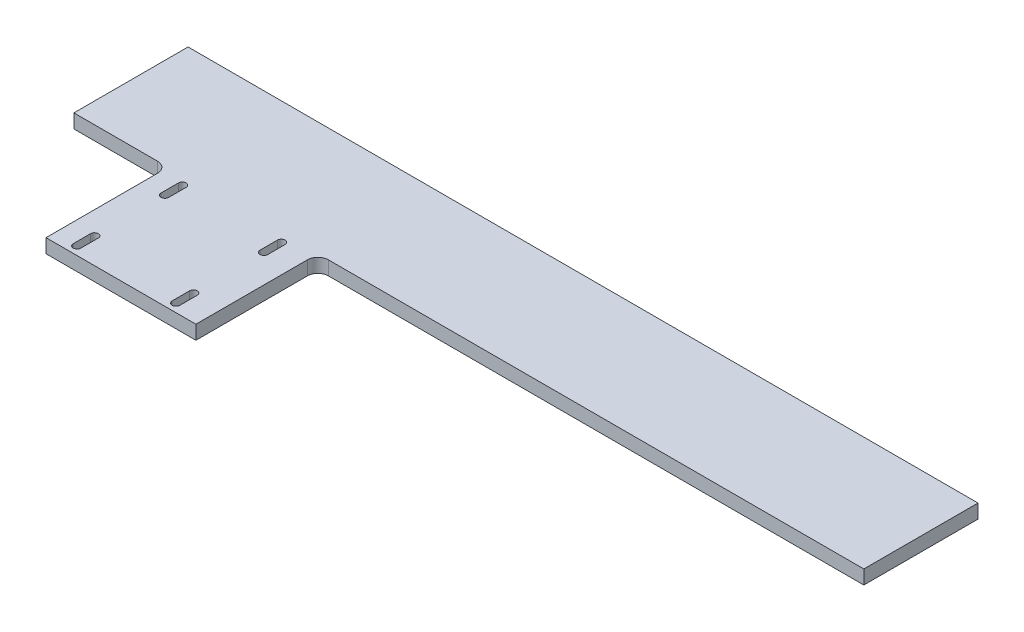
from build123d import *

# Parameters (mm, degrees)
SKETCH_1_W          = 2266
SKETCH_1_H          = 327.5
EXTRUDE_1_DEPTH     = 40
SKETCH_2_W          = 430
SKETCH_2_H          = 350
EXTRUDE_2_DEPTH     = 40
CUT_EXTRUDE_1_DEPTH = 1245.67990363
FILLET_1_R          = 30


with BuildPart() as part:
    # 草图1 → 凸台-拉伸1 (new body)
    with BuildSketch(Plane(origin=(0, 0, 0), x_dir=(1, 0, 0), z_dir=(0, 1, 0))):
        Rectangle(SKETCH_1_W, SKETCH_1_H)
    extrude(amount=EXTRUDE_1_DEPTH)

    # 草图2 → 凸台-拉伸2 (add)
    with BuildSketch(Plane(origin=(0, 40, 0), x_dir=(1, 0, 0), z_dir=(0, 1, 0))):
        with Locations((-648, -338.75)):
            Rectangle(SKETCH_2_W, SKETCH_2_H)
    extrude(amount=-EXTRUDE_2_DEPTH)

    # 草图3 → 切除-拉伸1 (cut, through all)
    with BuildSketch(Plane(origin=(0, 40, 0), x_dir=(1, 0, 0), z_dir=(0, 1, 0))):
        with BuildLine():
            Line((-503, -187.75), (-503, -237.75))
            ThreePointArc((-503, -237.75), (-514, -248.75), (-525, -237.75))
            Line((-525, -237.75), (-525, -187.75))
            ThreePointArc((-525, -187.75), (-514, -176.75), (-503, -187.75))
        make_face()
        with BuildLine():
            Line((-787, -187.75), (-787, -237.75))
            ThreePointArc((-787, -237.75), (-798, -248.75), (-809, -237.75))
            Line((-809, -237.75), (-809, -187.75))
            ThreePointArc((-809, -187.75), (-798, -176.75), (-787, -187.75))
        make_face()
        with BuildLine():
            Line((-787, -439.75), (-787, -489.75))
            ThreePointArc((-787, -489.75), (-798, -500.75), (-809, -489.75))
            Line((-809, -489.75), (-809, -439.75))
            ThreePointArc((-809, -439.75), (-798, -428.75), (-787, -439.75))
        make_face()
        with BuildLine():
            Line((-503, -439.75), (-503, -489.75))
            ThreePointArc((-503, -489.75), (-514, -500.75), (-525, -489.75))
            Line((-525, -489.75), (-525, -439.75))
            ThreePointArc((-525, -439.75), (-514, -428.75), (-503, -439.75))
        make_face()
    extrude(amount=-CUT_EXTRUDE_1_DEPTH, mode=Mode.SUBTRACT)

    # 圆角1
    fillet_1_edges = [part.edges().sort_by_distance(p)[0] for p in [
        (-433, 20, 163.75),
        (-863, 20, 163.75),
    ]]
    fillet(fillet_1_edges, radius=FILLET_1_R)


solid = part.part
